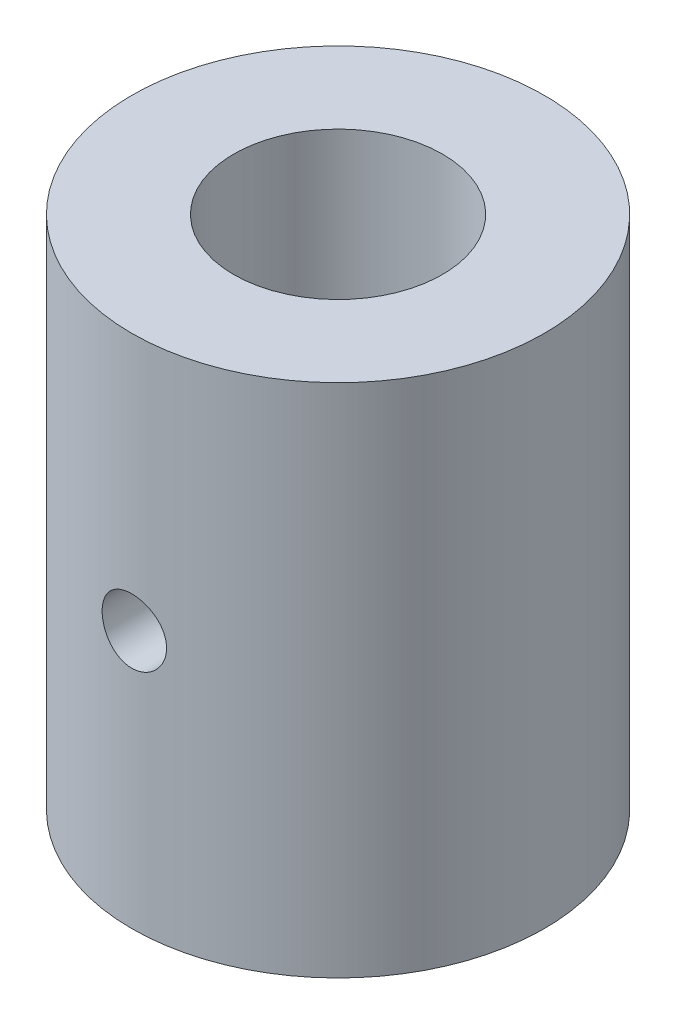
SolidWorks part; units mm, degrees
ref_plane "Front Plane" through (0, 0, 0) normal (0, 0, 1) x (1, 0, 0)
ref_plane "Top Plane" through (0, 0, 0) normal (0, 1, 0) x (1, 0, 0)
ref_plane "Right Plane" through (0, 0, 0) normal (1, 0, 0) x (0, 0, -1)
sketch "Sketch1" plane through (0, 0, 0) normal (0, 0, 1) x (1, 0, 0)
  line L0 (0, 29.6129) -> (0, 0) construction
  line L2 (4.05, 30.5161) -> (8, 30.5161)
  line L3 (4.05, 30.5161) -> (4.05, 10.5161)
  line L4 (4.05, 10.5161) -> (8, 10.5161)
  line L5 (8, 30.5161) -> (8, 10.5161)
  line L6 (4.05, 30.5161) -> (8, 10.5161) construction
  line L7 (4.05, 10.5161) -> (8, 30.5161) construction
  point P3 (6.025, 20.5161)
  dimension "D1" = 4.05
  dimension "D2" = 8
  dimension "D3" = 20
revolve "Revolve1" add sketch "Sketch1" angle 360 about L0
ref_plane "Plane1" through (0, 0, 8) normal (0, 0, 1) x (1, 0, 0)
sketch "Sketch4" plane through (0, 0, 8) normal (0, 0, 1) x (1, 0, 0)
  line L0 (0, 30.5161) -> (0, 10.5161) construction
  line L1 (8, 30.5161) -> (-8, 30.5161) construction
  line L2 (-8, 10.5161) -> (8, 10.5161) construction
  line L3 (0, 10.5161) -> (14.4687, 10.5161) construction
hole_wizard "M3 Tapped Hole1" positions "3DSketch1" profile "Sketch3" tap size "M3" standard "GB"
sketch3d "3DSketch1"
  line L0 (0, 30.5161, 8) -> (0, 10.5161, 8) construction
  line L1 (0, 10.5161, 8) -> (14.4687, 10.5161, 8) construction
  point P0 (0, 20.5161, 8)
  dimension "D1" = 10
sketch "Sketch3" plane through (0, 20.5161, 8) normal (1, 0, 0) x (0, -1, 0)
  line L0 (0, 0) -> (0, 3.95)
  line L1 (0, 3.95) -> (1.25, 3.95)
  line L2 (1.25, 3.95) -> (1.25, 0)
  line L5 (1.25, 0) -> (0, 0)
  line L11 (0, -6.35) -> (0, 107.95) construction
  dimension "通孔螺纹孔钻头直径" = 2.5
  dimension "通孔螺纹孔钻头深度" = 3.95
cosmetic thread "Cosmetic Thread3" parameters "D2"=3
